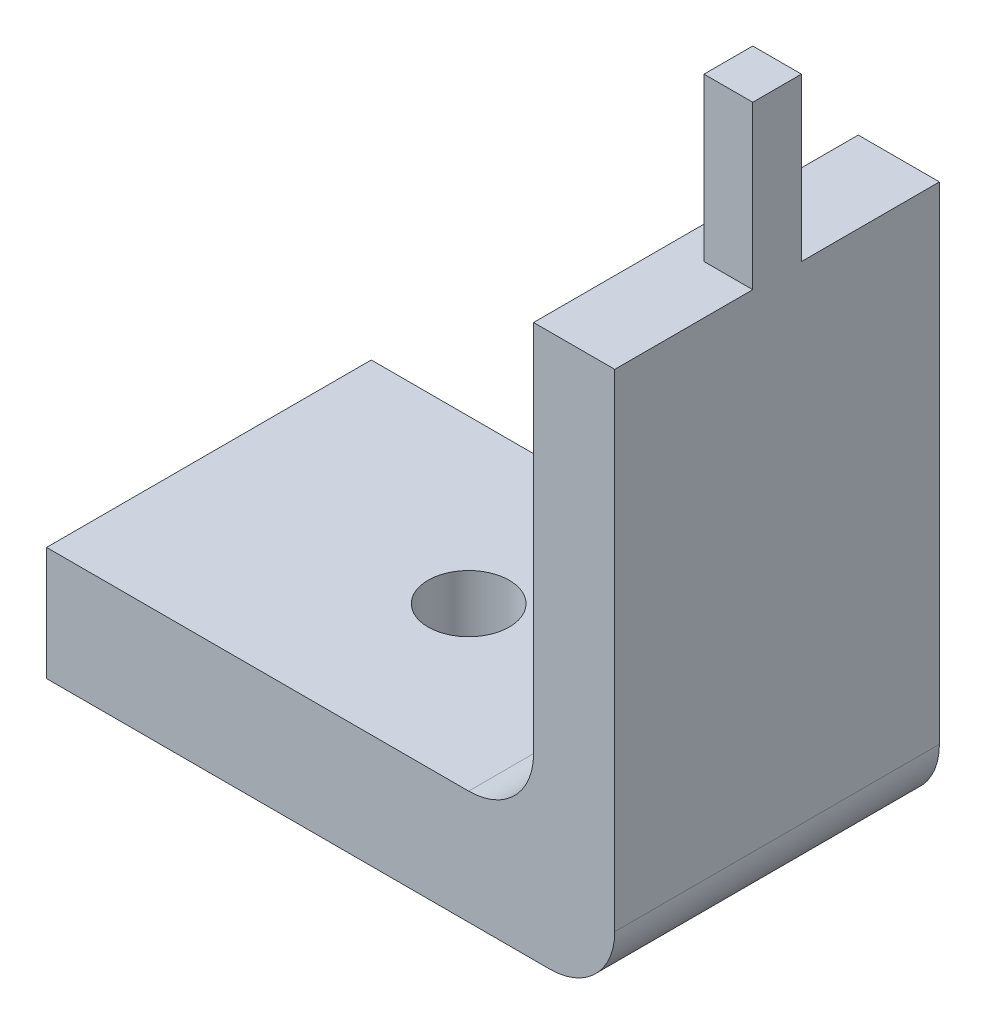
SolidWorks part; units mm, degrees
ref_plane "Front Plane" through (0, 0, 0) normal (0, 0, 1) x (1, 0, 0)
ref_plane "Top Plane" through (0, 0, 0) normal (0, 1, 0) x (1, 0, 0)
ref_plane "Right Plane" through (0, 0, 0) normal (1, 0, 0) x (0, 0, -1)
sketch "Sketch1" plane through (0, 0, 0) normal (0, 0, 1) x (1, 0, 0)
  line L5 (0, 0) -> (17.5, 0)
  line L6 (17.5, 0) -> (17.5, 17)
  line L8 (17.5, 17) -> (15, 17)
  line L9 (15, 17) -> (15, 3.5)
  line L10 (15, 3.5) -> (0, 3.5)
  line L11 (0, 3.5) -> (0, 0)
  dimension "D1" = 17.5
  dimension "D2" = 3.5
  dimension "D3" = 15
  dimension "D4" = 17
extrude "Boss-Extrude1" add sketch "Sketch1" along normal blind 10
sketch "Sketch2" plane through (17.5, 0, 0) normal (1, 0, 0) x (0, 0, -1)
  line L0 (-5.75, 17) -> (-5.75, 22)
  line L1 (-10, 17) -> (0, 17) construction
  line L2 (-5.75, 22) -> (-4.25, 22)
  line L3 (-4.25, 22) -> (-4.25, 17)
  line L4 (-5, 22) -> (-5, 17) construction
  line L5 (-5.75, 17) -> (-4.25, 17)
  dimension "D1" = 1.5
  dimension "D2" = 5
extrude "Boss-Extrude2" add sketch "Sketch2" against normal blind 1.5
fillet "Fillet1" radius 2 2 edges at (15, 3.5, 5) (17.5, 0, 5)
hole_wizard "M3 Tapped Hole1" positions "Sketch3" profile "Sketch4" tap size "M3" standard "GB"
sketch "Sketch3" plane through (0, 3.5, 0) normal (0, 1, 0) x (1, 0, 0)
  line L0 (0, -10) -> (0, 0) construction
  line L1 (13, -10) -> (0, -10) construction
  point P0 (8, -5)
  dimension "D1" = 8
  dimension "D2" = 5
sketch "Sketch4" plane through (8, 3.5, 5) normal (1, 0, 0) x (0, 0, 1)
  line L0 (0, 0) -> (0, 9.2511)
  line L1 (0, 9.2511) -> (1.25, 8.5)
  line L2 (1.25, 8.5) -> (1.25, 0)
  line L5 (1.25, 0) -> (0, 0)
  line L10 (0, 9.2511) -> (-1.25, 8.5) construction
  line L11 (0, -6.35) -> (0, 107.95) construction
  dimension "螺纹孔钻头直径" = 2.5
  dimension "螺纹孔钻头深度" = 8.5
  dimension "导头角度" = 118
cosmetic thread "Cosmetic Thread1" parameters "D1"=6, "D2"=3
equation "\"1\"= \"代号代号\""
equation "\"2\"= \"名称代号\""
